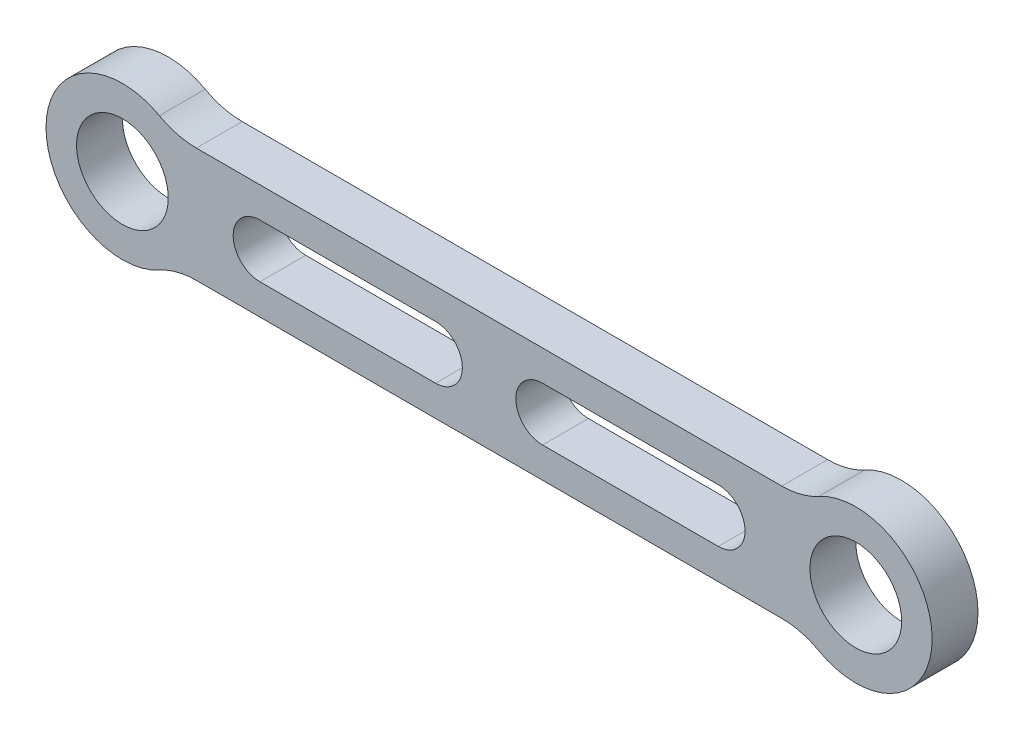
from build123d import *

# Parameters (mm, degrees)
SKETCH_1_R      = 6
EXTRUDE_1_DEPTH = 6
FILLET_R10_1_R  = 10


with BuildPart() as part:
    # 草图1 → 凸台-拉伸1 (new body)
    with BuildSketch(Plane.XY):
        with BuildLine():
            Line((6.614378278, 7.5), (89.385621722, 7.5))
            ThreePointArc((89.385621722, 7.5), (106, 0), (89.385621722, -7.5))
            Line((89.385621722, -7.5), (6.614378278, -7.5))
            ThreePointArc((6.614378278, -7.5), (-10, 0), (6.614378278, 7.5))
        make_face()
        Circle(SKETCH_1_R, mode=Mode.SUBTRACT)
        with Locations((96, 0)):
            Circle(SKETCH_1_R, mode=Mode.SUBTRACT)
        with BuildLine():
            Line((18, 3.5), (41, 3.5))
            ThreePointArc((41, 3.5), (44.5, 0), (41, -3.5))
            Line((41, -3.5), (18, -3.5))
            ThreePointArc((18, -3.5), (14.5, 0), (18, 3.5))
        make_face(mode=Mode.SUBTRACT)
        with BuildLine():
            Line((78, -3.5), (55, -3.5))
            ThreePointArc((55, -3.5), (51.5, 0), (55, 3.5))
            Line((55, 3.5), (78, 3.5))
            ThreePointArc((78, 3.5), (81.5, 0), (78, -3.5))
        make_face(mode=Mode.SUBTRACT)
    extrude(amount=EXTRUDE_1_DEPTH)

    # R10 圆角1
    fillet_r10_1_edges = [part.edges().sort_by_distance(p)[0] for p in [
        (6.614378278, 7.5, 3),
        (89.385621722, 7.5, 3),
        (89.385621722, -7.5, 3),
        (6.614378278, -7.5, 3),
    ]]
    fillet(fillet_r10_1_edges, radius=FILLET_R10_1_R)


solid = part.part
